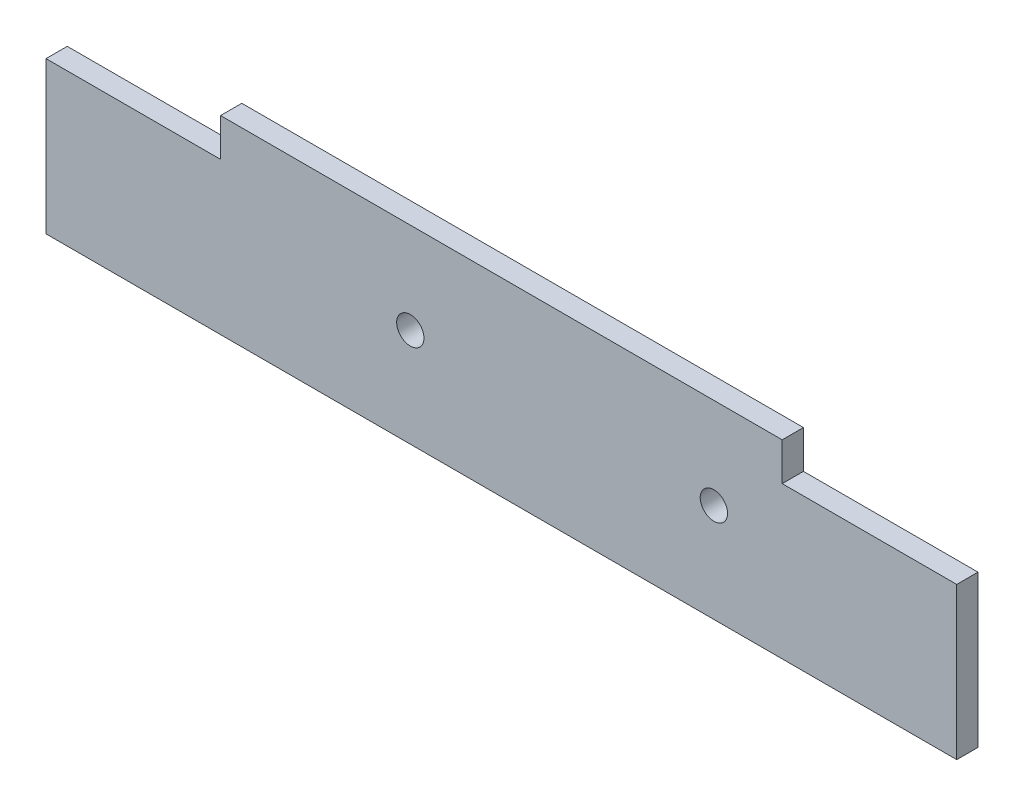
SolidWorks part; units mm, degrees
material "普通碳钢"
ref_plane "前视基准面" through (0, 0, 0) normal (0, 0, 1) x (1, 0, 0)
ref_plane "上视基准面" through (0, 0, 0) normal (0, 1, 0) x (1, 0, 0)
ref_plane "右视基准面" through (0, 0, 0) normal (1, 0, 0) x (0, 0, -1)
sketch "草图1" plane through (0, 0, 0) normal (0, 0, 1) x (1, 0, 0)
  line L0 (0, 0) -> (0, 100)
  line L1 (0, 100) -> (115, 100)
  line L2 (115, 100) -> (115, 125)
  line L3 (115, 125) -> (485, 125)
  line L4 (485, 125) -> (485, 100)
  line L5 (485, 100) -> (600, 100)
  line L6 (600, 100) -> (600, 0)
  line L7 (600, 0) -> (0, 0)
  circle A0 centre (240, 65) radius 9
  circle A1 centre (440, 65) radius 9
  dimension "D8" = 18
  dimension "D1" = 370
  dimension "D2" = 600
  dimension "D3" = 25
  dimension "D4" = 100
  dimension "D5" = 160
  dimension "D6" = 200
  dimension "D7" = 60
extrude "凸台-拉伸1" add sketch "草图1" along normal blind 14
